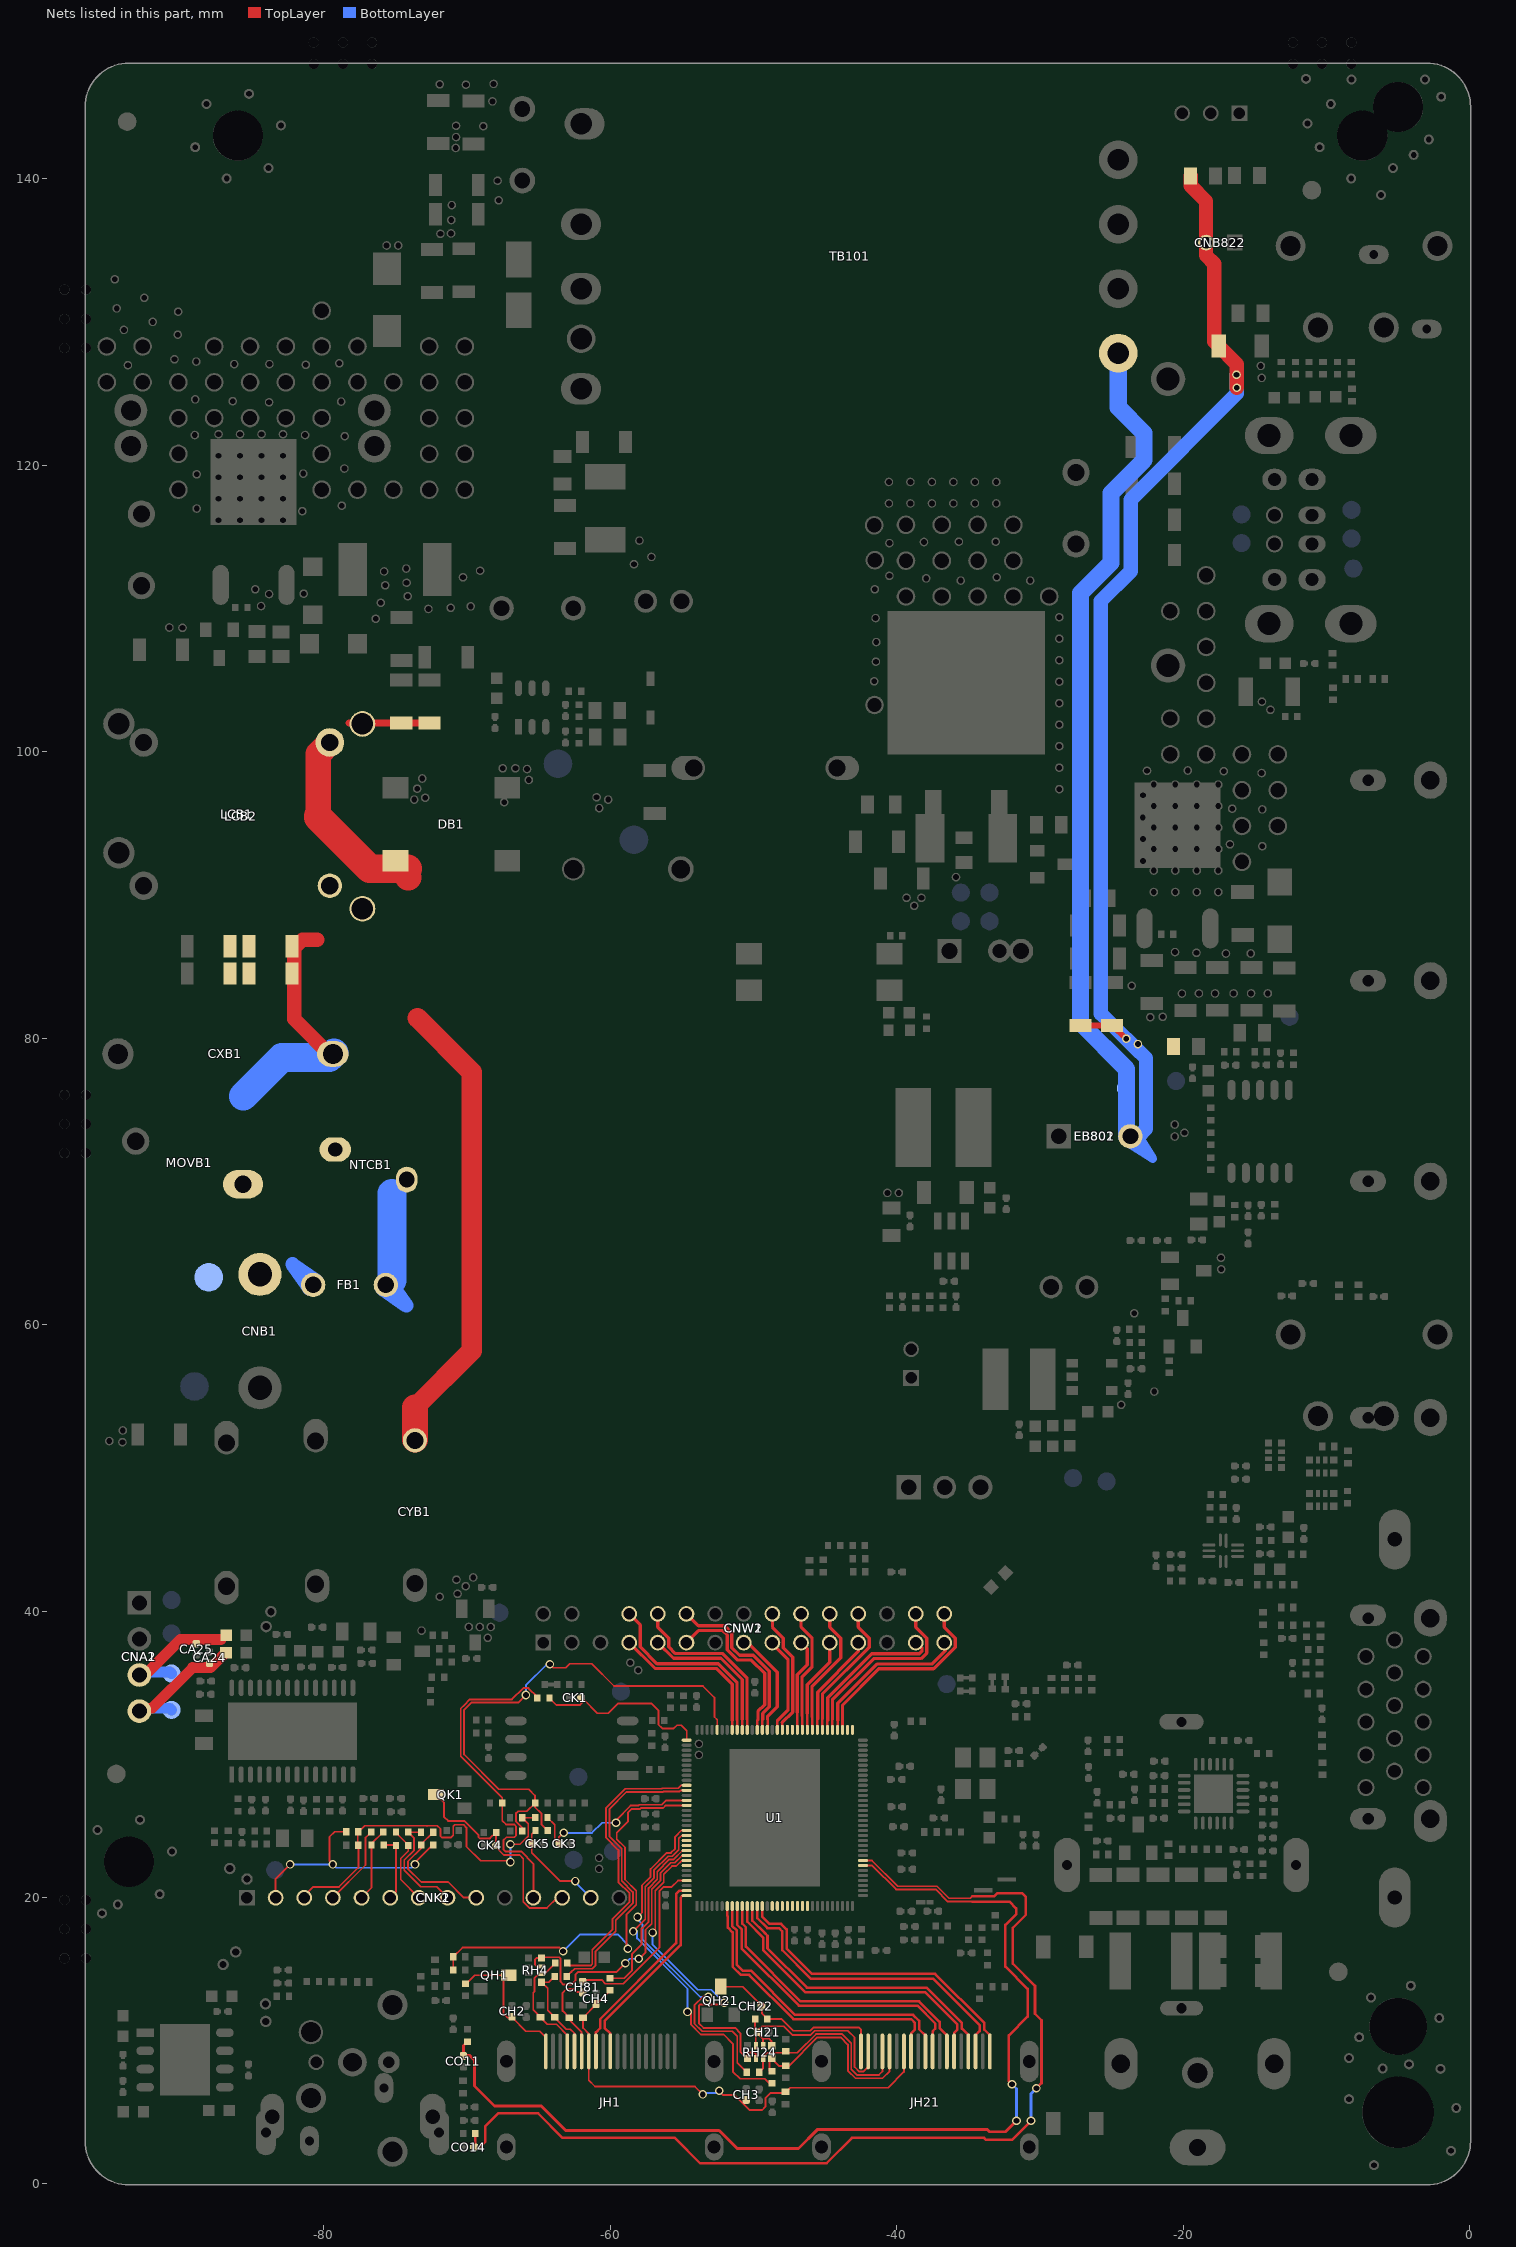
[diagram p0: the nets of this part, all layers, seen from the top]
# Altium PCB MISC86372.PcbDoc (part 11 of 16)
Units mm, origin at the board's own origin, x right, y up, seen from the top; angles counter-clockwise.
Board outline 96.73 x 148.13 mm, 2 copper layers (TopLayer, BottomLayer), stack 1.571 mm thick; 578 components, 318 nets, 2702 pads, 836 vias.

## Via types
v1: diameter 0.6, hole 0.4, TopLayer to BottomLayer, tented both sides, 816 vias
v2: diameter 0.7, hole 0.5, TopLayer to BottomLayer, tented both sides, 15 vias
v3: diameter 0.8, hole 0.5, TopLayer to BottomLayer, tented both sides, 5 vias

## Nets (pads, with @x,y where several pads share a name; then routed paths per layer and width w, separated by ;. In a path a pad name is that pad's centre, name@x,y a point inside that pad or via, vN(x,y) a via of type N, cw(c..) or ccw(c..) an arc to the next point about the centre after c; other vN are vias at no path point) (continued)
HDMI_A_CKN_IN_IC: JH1.12 U1.127 | length 14.1
  TopLayer w0.178: JH1.12@-61,9.258 -61,10.577 -60.706,10.871 -60.706,11.502 -55.397,16.81 -55.397,20.247 -55.188,20.456 -54.687,20.456 U1.127@-54.663,20.481
HDMI_A_CKP_IN_IC: JH1.10 U1.128 | length 13.6
  TopLayer w0.178: JH1.10@-60,9.258 -60,10.495 -60.401,10.897 -60.401,11.375 -55.093,16.684 -55.093,19.981 -54.943,20.131 U1.128@-54.663,20.131
HDMI_A_HPD_OUT: CH2.1 JH1.19 QH1.C RH3.1 | length 10.2
  TopLayer w0.127: RH3.1@-70.098,13.931 -69.463,14.567 QH1.C@-67.081,14.567 ; QH1.C@-67.462,14.185 -67.462,11.911 -67.18,11.628 -66.861,11.628 -65.898,10.665 -64.919,10.665 -64.5,10.247 JH1.19@-64.5,9.258
HDMI_A_HPD_OUT_IC: RH4.2 RH4.4 U1.120 | length 20
  TopLayer w0.127: RH4.4@-64.803,15.185 -65.122,15.185 -65.253,15.316 -65.253,15.676 -65.144,15.785 RH4.2@-64.803,15.785 RH4.2@-64.803,15.909 ; RH4.2@-64.803,15.833 -63.562,15.833 -63.465,15.736 -63.465,14.113 -63.271,13.919 -62.713,13.919 -62.433,14.199 -62.433,14.605 -62.236,14.802 -59.555,14.802 v1(-58.942,15.414) ; v1@-57.991,15.703 -57.551,16.143 -57.551,17.729 -57.099,18.181 -57.099,20.566 -56.497,21.167 -56.497,21.704 -55.775,22.427 -55.488,22.427 -54.984,22.931 U1.120@-54.613,22.931
  BottomLayer w0.127: v1(-58.942,15.414) -58.634,15.723 -58.014,15.723 v1(-58.012,15.724)
HDMI_A_SCL_IN: DH2.K JH1.15 RH4.8 RH6.1 | length 7.1
  TopLayer w0.127: RH6.1@-63.874,14.494 -64.283,14.085 RH4.8@-64.803,14.085 -64.371,13.654 -64.371,12.131 DH2.K@-63.881,11.64 -63.881,11.601 -63.081,10.801 -62.783,10.801 -62.5,10.518 JH1.15@-62.5,9.258
HDMI_A_SCL_IN_IC: RH6.2 U1.107 | length 21.1
  TopLayer w0.127: RH6.2@-63.024,14.494 -62.712,14.807 ; -62.564,14.954 -62.712,14.807 ; U1.107@-54.664,27.481 -55.085,27.481 -55.169,27.397 -56.284,27.397 -56.318,27.364 -58.875,27.364 -60.063,26.175 -60.063,24.265 -59.201,23.403 -59.201,21.161 -58.421,20.381 -58.421,19.599 -59.623,18.397 -59.623,17.655 -61.025,16.252 -61.025,15.261 -61.256,15.03 -62.488,15.03 -62.712,14.807
HDMI_A_SDA_IO: DH3.K JH1.16 RH4.6 RH5.1 | length 8.3
  TopLayer w0.127: RH4.6@-64.99,14.685 -65.287,14.387 -65.287,13.45 -65.38,13.358 -65.38,12.159 DH3.K@-64.861,11.64 ; DH3.K@-64.897,11.645 -64.403,11.151 -63.754,11.151 -63,10.397 JH1.16@-63,9.258 ; RH4.6@-64.803,14.685 -64.587,14.685 RH5.1@-63.855,15.418 RH5.1@-63.932,15.418
HDMI_A_SDA_IO_IC: RH5.2 U1.106 | length 20.8
  TopLayer w0.127: RH5.2@-63.005,15.418 -62.846,15.259 -61.35,15.259 -61.254,15.356 -61.254,16.347 -59.851,17.749 -59.851,18.492 -58.649,19.694 -58.649,20.286 -59.43,21.066 -59.43,23.308 -60.292,24.17 -60.292,26.27 -58.969,27.592 -56.412,27.592 -56.379,27.626 -55.263,27.626 -55.059,27.831 U1.106@-54.664,27.831 ; U1.106@-54.673,27.821 U1.106@-54.663,27.831
HDMI_ARC_OUT: CH81.1 DH81.K JH1.14 | length 6.1
  TopLayer w0.127: DH81.K@-62.865,11.455 -62,10.59 JH1.14@-62,9.258 ; DH81.K@-62.865,11.615 -63.33,12.08 -63.33,13.35 -63.058,13.622 -62.535,13.622 -62.306,13.393 CH81.1@-61.946,13.393
HDMI_ARC_OUT_IC: CH81.2@-61.925,13.995 CH81.2@-61.925,14.17 U1.125 | length 12.7
  TopLayer w0.127: CH81.2@-61.946,14.243 -60.609,14.243 -60.339,13.973 -59.106,13.973 -56.553,16.526 -56.553,20.466 -56.279,20.739 -55.715,20.739 -55.273,21.181 U1.125@-54.663,21.181
HDMI_B_0N_IN_IC: JH21.9 U1.9 | length 20.8
  TopLayer w0.178: U1.9@-51.138,19.406 -51.138,18.099 -50.837,17.797 -50.837,16.451 -46.831,12.446 -38.568,12.446 -37.313,11.191 -37.313,10.846 -37.5,10.658 JH21.9@-37.5,9.258 JH21.9@-37.49,9.267
HDMI_B_0P_IN_IC: JH21.7 U1.10 | length 20.9
  TopLayer w0.178: U1.10@-50.788,19.406 -50.788,18.18 -50.532,17.924 -50.532,16.578 -46.705,12.751 -38.441,12.751 -37.008,11.317 -37.008,10.878 -36.5,10.37 JH21.7@-36.5,9.258 JH21.7@-36.525,9.283
HDMI_B_1N_IN_IC: JH21.6 U1.11 | length 21.2
  TopLayer w0.178: U1.11@-50.438,19.406 -50.438,18.312 -49.33,17.204 -49.33,16.328 -46.401,13.399 -38.036,13.399 -35.763,11.126 -35.763,10.77 -36,10.533 JH21.6@-36,9.258
HDMI_B_1P_IN_IC: JH21.4 U1.12 | length 21.3
  TopLayer w0.178: U1.12@-50.088,19.406 -50.088,18.393 -49.204,17.508 -49.025,17.33 -49.025,16.454 -46.274,13.703 -37.91,13.703 -35.458,11.252 -35.458,10.846 -35,10.387 JH21.4@-35,9.258
HDMI_B_2N_IN_IC: JH21.3 U1.13 | length 22.2
  TopLayer w0.178: U1.13@-49.738,19.406 -49.738,18.569 -49.025,17.856 -48.208,17.856 -47.993,17.641 -47.993,16.32 -46.011,14.338 -37.46,14.338 -34.214,11.092 -34.214,10.671 -34.5,10.385 JH21.3@-34.5,9.258
HDMI_B_2P_IN_IC: JH21.1 U1.14 | length 22.2
  TopLayer w0.178: U1.14@-49.388,19.406 -49.388,18.65 -48.899,18.161 -48.082,18.161 -47.688,17.767 -47.688,16.447 -45.91,14.668 -37.323,14.668 -33.884,11.229 -33.884,10.768 -33.5,10.385 JH21.1@-33.5,9.258
HDMI_B_5V: CH21.1 JH21.18 RH23.2 RH24.4 RH24.6 RH24.8 | length 16.1
  TopLayer w0.127: RH23.2@-49.888,11.527 -49.888,10.74 CH21.1@-49.738,10.59 ; RH24.4@-49.85,9.649 -49.85,10.349 CH21.1@-49.676,10.523 ; CH21.1@-49.809,10.519 CH21.1@-49.738,10.59 ; CH21.1@-49.738,10.394 CH21.1@-49.738,10.59 ; CH21.1@-49.738,10.656 -49.389,11.006 -47.886,11.006 -47.275,10.394 -46.031,10.394 -45.732,10.693 -43.409,10.693 -42.951,10.236 -42.951,8.172 -42.622,7.842 -42.348,7.842 -42,8.19 JH21.18@-42,9.258 ; CH21.1@-49.605,10.398 -49.346,10.138 ; CH21.1@-49.563,10.59 CH21.1@-49.479,10.506 ; RH24.6@-49.35,9.649 -49.346,9.653 -49.346,10.138 ; RH24.8@-48.75,9.649 -48.75,9.974 -48.914,10.138 -49.346,10.138
HDMI_B_CKN_IN_IC: JH21.12 U1.7 | length 20.8
  TopLayer w0.178: U1.7@-51.838,19.406 -51.838,18.734 -51.793,18.689 -51.793,17.892 -51.46,17.559 -51.46,15.164 -50.887,14.591 -50.306,14.591 -47.22,11.506 -38.988,11.506 -38.735,11.253 -38.735,10.77 -39,10.505 JH21.12@-39,9.258
HDMI_B_CKP_IN_IC: JH21.10 U1.8 | length 20.9
  TopLayer w0.178: U1.8@-51.488,19.406 -51.488,18.018 -51.156,17.685 -51.156,15.291 -50.761,14.896 -50.179,14.896 -47.094,11.811 -38.862,11.811 -38.43,11.379 -38.43,10.797 -38,10.367 JH21.10@-38,9.258
HDMI_B_HPD_OUT: CH22.1 JH21.19 QH21.C RH23.1 | length 14.6
  TopLayer w0.127: QH21.C@-52.286,13.768 -50.75,13.768 CH22.1@-49.403,12.421 -49.403,11.892 RH23.1@-49.038,11.527 -48.068,11.527 -47.236,10.696 -46.053,10.696 -45.826,10.922 -45.288,10.922 ; -45.593,10.922 -45.288,10.922 ; JH21.19@-42.5,10.471 JH21.19@-42.5,9.258 -42.5,10.795 -42.627,10.922 -45.288,10.922
HDMI_B_HPD_OUT_IC: RH24.1 RH24.3 U1.121 | length 23.6
  TopLayer w0.127: v1@-56.865,17.551 -56.865,20.477 -56.269,21.073 -56.269,21.61 -55.68,22.198 -55.393,22.198 -55.011,22.581 U1.121@-54.613,22.581 ; v1@-52.007,12.649 v1(-52.045,12.649) -52.045,12.537 -52.056,12.525 -53.75,12.525 -53.816,12.459 -53.816,11.217 -53.491,10.892 -51.278,10.892 -50.913,10.527 -50.913,9.232 RH24.1@-50.43,8.749 -50.43,9.117 -50.374,9.173 -49.905,9.173 -49.83,9.099 RH24.3@-49.83,8.749
  BottomLayer w0.127: v1(-57.048,17.551) -57.048,16.711 -53.901,13.564 -52.959,13.564 v1(-52.045,12.649)
HDMI_B_SCL_IN: DH22.K JH21.15 RH24.7 RH26.1 | length 14.1
  TopLayer w0.127: RH24.7@-48.883,8.745 -48.883,7.87 RH26.1@-48.793,7.78 ; RH24.7@-48.75,8.749 RH24.7@-48.73,8.749 -48.215,8.233 -47.756,8.233 -47.752,8.23 -47.549,8.23 -45.542,10.236 -43.91,10.236 -43.409,9.735 -43.409,7.913 -42.881,7.385 -40.997,7.385 -40.5,7.882 JH21.15@-40.5,9.258
HDMI_B_SCL_IN_IC: RH26.2 U1.116 | length 25.2
  TopLayer w0.127: v1(-58.395,17.63) -57.556,18.468 -57.556,20.755 -56.955,21.357 -56.955,21.894 -55.964,22.884 -55.677,22.884 -55.22,23.341 -55.22,24.127 -55.016,24.331 U1.116@-54.663,24.331 ; v1@-54.356,11.9 -54.356,11.11 -53.68,10.435 -52.076,10.435 -51.435,9.794 -51.435,7.846 -50.929,7.341 -49.204,7.341 RH26.2@-48.793,6.93
  BottomLayer w0.127: v1(-58.395,17.63) -58.129,17.63 -58.129,17.145 -54.61,13.626 v1(-54.61,12.014)
HDMI_B_SDA_IO: DH23.K JH21.16 RH24.5 RH25.1 | length 13.9
  TopLayer w0.127: RH25.1@-49.613,7.798 -49.33,8.081 RH24.5@-49.33,8.749 -49.33,8.882 -49.049,9.164 -46.946,9.164 -46.942,9.16 -45.637,10.465 -43.815,10.465 -43.18,9.83 -43.18,8.008 -42.786,7.614 -41.241,7.614 -41,7.855 JH21.16@-41,9.258
HDMI_B_SDA_IO_IC: RH25.2 U1.115 | length 24.2
  TopLayer w0.127: v1(-58.092,18.642) -57.785,18.948 -57.785,20.85 -57.183,21.452 -57.183,21.989 -56.059,23.113 -55.772,23.113 -55.474,23.411 -55.474,24.232 -55.026,24.681 U1.115@-54.663,24.681 ; v1@-53.365,13.106 -53.492,13.106 -54.127,12.471 -54.127,11.205 -53.586,10.663 -51.481,10.663 -51.142,10.324 -51.142,8.477 RH25.2@-50.463,7.798
  BottomLayer w0.127: v1(-58.092,18.642) -58.092,18.468 -57.76,18.136 -57.76,17.099 -53.716,13.056 v1(-53.162,13.056)
HDMI_C_0N_IN_IC: U1.18
HDMI_C_0P_IN_IC: U1.19
HDMI_C_1N_IN_IC: U1.20
HDMI_C_1P_IN_IC: U1.21
HDMI_C_2N_IN_IC: U1.22
HDMI_C_2P_IN_IC: U1.23
HDMI_C_CKN_IN_IC: U1.16
HDMI_C_CKP_IN_IC: U1.17
HDMI_C_HPD_OUT_IC: U1.122
HDMI_C_SCL_IN_IC: U1.118
HDMI_C_SDA_IO_IC: U1.117
HDMI_CEC_IO: CH3.2@-50.506,5.819 CH3.2@-50.506,5.994 CH4.2@-61.006,12.503 CH4.2@-61.006,12.678 DH1.K DH21.K JH1.13 JH21.13 RH83.2 | length 34.3
  TopLayer w0.127: CH4.2@-61.006,12.503 -60.02,13.489 RH83.2@-60.02,13.513 ; CH4.2@-61.006,12.515 DH1.K@-61.906,11.615 -61.906,10.895 -61.5,10.489 JH1.13@-61.5,9.258 -61.5,7.239 -61.068,6.807 -54.092,6.807 v1(-53.538,6.253) ; v1@-52.4,6.477 -52.146,6.223 -51.353,6.223 -50.301,5.171 -49.397,5.171 -49.393,5.167 -49.174,5.386 -49.174,5.989 -48.822,6.342 -47.802,6.342 -47.422,6.722 -40.598,6.722 -39.5,7.82 JH21.13@-39.5,9.258 JH21.13@-39.5,10.392
  BottomLayer w0.127: v1(-53.538,6.253) -53.441,6.35 -52.553,6.35 v1(-52.4,6.502)
HDMI_CEC_IO_IC: RH83.1 U1.119 | length 12.1
  TopLayer w0.127: RH83.1@-60.02,14.363 -59.039,14.363 -58.477,14.924 -58.477,16.06 -57.81,16.727 -57.81,17.831 -57.328,18.313 -57.328,20.66 -56.726,21.262 -56.726,21.799 -55.87,22.656 -55.583,22.656 -54.958,23.281 U1.119@-54.613,23.281
HDMI_DET: RH81.1 RH82.1 U1.110 | length 29.5
  TopLayer w0.127: RH82.1@-70.961,15.861 -70.312,16.51 -63.551,16.51 ; RH82.1@-70.923,15.823 -70.961,15.785 RH81.1@-70.961,14.935 ; -63.525,16.51 -63.551,16.51 ; v1(-63.297,16.256) -63.551,16.51 ; v1@-58.86,16.516 -58.86,18.837 -58.192,19.504 -58.192,20.475 -58.972,21.256 -58.972,23.497 -59.55,24.075 -59.55,24.519 -58.768,25.3 -58.768,25.914 -58.496,26.187 -57.914,26.187 -57.853,26.247 -56.298,26.247 -56.114,26.431 U1.110@-54.664,26.431 ; RH81.1@-70.961,14.935 -70.961,14.884 RH81.1@-70.961,14.935
  BottomLayer w0.127: v1@-63.246,16.29 -62.111,17.424 -59.493,17.424 -58.769,16.701 v1(-58.769,16.426)
IR_IN: CNK1.11 CNK2.11 RK1.1 RK2.1 | length 24.2
  TopLayer w0.127: -67.749,27.17 -68.162,27.584 ; CNK2.11@-65.365,19.99 -65.365,22.362 -66.222,23.22 -67.322,23.22 -67.462,23.36 -67.462,23.991 -67.246,24.207 -66.694,24.207 -66.583,24.319 -66.583,24.971 -66.717,25.104 -67.279,25.104 -67.545,25.371 RK1.1@-67.545,26.594 -67.545,26.967 -68.162,27.584 ; RK2.1@-65.093,33.925 -65.093,34.001 -65.712,34.62 -66.077,34.62 -66.865,33.833 -68.274,33.833 -68.275,33.831 -69.801,33.831 -70.21,33.422 -70.437,33.195 -70.437,29.858 -68.162,27.584
IR_IN_IC: CK1.2@-62.014,33.941 CK1.2@-62.189,33.941 RK2.2 U1.97 | length 12.9
  TopLayer w0.127: RK2.2@-64.243,33.925 -63.753,33.435 -62.122,33.435 -62.014,33.543 -62.014,33.905 CK1.2@-62.014,33.941 ; CK1.2@-61.836,33.801 -60.902,32.868 -60.138,32.868 -59.452,33.553 -57.134,33.553 -56.642,33.062 -56.642,32.076 -56.367,31.801 -55.573,31.801 -55.344,32.029 -55.044,32.029 -54.664,31.649 U1.97@-54.664,30.981
K0: CNK1.9 CNK2.9 RK7.1 RK8.2 | length 8.8
  TopLayer w0.127: RK7.1@-73.225,23.7 RK8.2@-72.366,24.559 ; RK7.1@-73.207,23.663 -73.207,23.431 -74.126,22.512 -74.126,22.012 -73.196,21.082 -71.323,21.082 -70.231,19.99 CNK2.9@-69.365,19.99
K1: CNK1.8 CNK2.8 RK8.1 RK9.2 | length 7.8
  TopLayer w0.127: RK9.2@-74.11,24.567 RK9.2@-74.102,24.559 ; RK8.1@-73.216,24.559 RK9.2@-74.102,24.559 ; CNK2.8@-71.365,19.99 -72.127,20.752 -73.225,20.752 -74.38,21.906 -74.38,22.617 -73.694,23.303 -73.694,24.151 RK9.2@-74.102,24.559
K2: CNK1.7 CNK2.7 RK9.1 RK11.2 | length 5.7
  TopLayer w0.127: RK9.1@-74.96,24.567 -74.96,24.508 RK11.2@-74.085,23.633 ; RK11.2@-74.109,23.641 -74.109,23.247 -74.634,22.723 -74.634,21.259 CNK2.7@-73.365,19.99
K3: CNK1.6 CNK2.6 RK11.1 RK12.2 | length 4.8
  TopLayer w0.127: RK12.2@-75.821,23.658 RK11.1@-74.997,23.658 ; CNK2.6@-75.365,19.99 -74.959,20.395 RK11.1@-74.959,23.743 ; RK11.1@-74.97,23.631 RK11.1@-74.959,23.62
K4: CNK1.5 CNK2.5 RK12.1 RK16.2 | length 5.3
  TopLayer w0.127: CNK2.5@-77.365,19.99 -76.671,20.683 RK12.1@-76.671,23.76 ; RK12.1@-76.675,23.658 -76.675,23.748 RK16.2@-75.85,24.573
K5: CNK1.4 CNK2.4 RK16.1 | length 5.7
  TopLayer w0.127: CNK2.4@-79.365,19.99 -77.087,22.268 -77.087,24.186 RK16.1@-76.7,24.573
K6: CNK1.3 CNK2.3 DK1.K RK3.1 RK4.2 RK6.2 | length 26.4
  TopLayer w0.127: CNK2.3@-81.365,19.99 -81.365,20.108 -80.734,20.739 -78.939,20.739 -77.585,22.093 DK1.K@-77.585,23.648 ; DK1.K@-77.627,23.582 -77.627,24.539 -77.152,25.013 -72.806,25.013 ; -72.773,24.999 -72.792,24.999 -72.806,25.013 ; v1@-66.972,22.563 -69.053,22.563 -70.036,23.546 -70.04,23.546 -70.04,24.881 -70.243,25.084 -70.861,25.084 -70.958,24.987 -70.958,24.343 -71.107,24.194 -71.753,24.194 -71.851,24.292 -71.851,24.789 -72.076,25.013 -72.806,25.013 ; v1(-66.972,23.717) -66.301,23.717 -65.733,24.285 -65.733,25.152 RK3.1@-66.15,25.569 -65.249,25.569 RK4.2@-65.233,25.585
  BottomLayer w0.127: v1(-66.972,22.475) v1(-66.972,23.717)
K7: CNK1.2 CNK2.2 RK6.1 RK7.2 | length 17.2
  TopLayer w0.127: CNK2.2@-83.138,19.99 CNK2.2@-83.365,19.99 -83.365,21.296 v1(-82.352,22.309) ; v1(-79.367,22.309) -79.604,22.546 -79.604,24.232 -79.24,24.595 RK6.1@-78.433,24.595 ; v1@-73.661,22.322 -73.661,22.42 RK7.2@-72.327,23.754
  BottomLayer w0.127: v1(-82.352,22.309) v1(-79.367,22.309) -79.131,22.073 -73.872,22.073 v1(-73.635,22.309)
KEY_IN_IC: CK3.2@-63.42,23.749 CK3.2@-63.595,23.749 RK4.1 U1.109 | length 12.5
  TopLayer w0.127: RK4.1@-64.383,25.585 -63.881,25.082 -63.881,24.035 CK3.2@-63.595,23.749 -63.595,24.218 v1@-63.274,24.539 ; v1@-59.598,25.408 -58.591,26.415 -58.034,26.415 -57.973,26.475 -56.392,26.475 -56.087,26.781 U1.109@-54.664,26.781
  BottomLayer w0.127: v1(-63.246,24.511) -61.28,24.511 -60.57,25.221 v1(-59.598,25.221)
L: CYB1.1 DB1.2 LCB1.3 LCB2.3 RB101.1 RB141.2 | length 51.6
  TopLayer w0.5: -78.224,101.989 -78.208,102.005 RB141.2@-72.619,102.005
  TopLayer w1.4: -73.635,54.204 -69.672,58.166 -69.672,77.622 -73.457,81.407
  TopLayer w1.8: -80.391,95.504 -80.391,99.822 LCB1.3@-79.578,100.635 ; -74.131,91.201 -74.08,91.201 ; CYB1.1@-73.635,51.968 -73.635,54.204
  TopLayer w2: -80.391,95.504 -80.391,95.409 -76.793,91.811 DB1.2@-74.131,91.811
L-1: CNB1.1 FB1.1 TP_L.1
L-2: FB1.2 NTCB1.1 | length 6.1
  BottomLayer w2: FB1.2@-75.235,63.094 -75.235,69.164
L-3: CXB1.1 LCB1.2 LCB2.2 MOVB1.1 NTCB1.2@-79.208,72.221 RB1.1 RB2.1 | length 18.3
  TopLayer w1: -80.467,86.868 -81.483,86.868 -82.067,86.284 -82.067,81.331 CXB1.1@-79.299,78.562
  BottomLayer w2: -85.633,75.937 -82.931,78.638 -79.622,78.638 CXB1.1@-79.292,78.969
L-N: RB1.2 RB2.2 RB3.1 RB4.1
LED_FB: CB808.2 CNB822.2 EB801.2 EB802.2@-23.687,73.139 pad.VIA5@-16.256,125.4 pad.VIA5@-16.281,126.314 pad.VIA5@-23.165,79.578 pad.VIA5@-23.978,79.959 RB814.1 RB825.2 RB826.2 RB845.1 TB101.7 TP_LED-.1 | length 138.8
  TopLayer w0.4: RB826.2@-27.178,80.796 -27.102,80.872 RB825.2@-24.968,80.872 pad.VIA5@-23.978,79.959
  TopLayer w1: RB845.1@-19.484,140.183 -19.484,139.499 -18.408,138.423 CNB822.2@-18.408,135.534 -18.408,135.299 -18.408,134.639 -17.831,134.061 -17.831,128.623 CB808.2@-17.527,128.32 -16.256,127.048 pad.VIA5@-16.256,125.4
  BottomLayer w1: pad.VIA5@-23.978,79.959 -22.606,78.588 -22.606,73.66 -23.113,73.153 -23.127,73.139 EB801.2@-23.687,73.139 ; -23.087,79.039 -25.756,81.708 -25.756,110.515 -23.673,112.598 -23.673,117.577 -16.256,124.993 pad.VIA5@-16.256,125.4 pad.VIA5@-16.256,126.314
  BottomLayer w1.2: TB101.7@-24.538,127.819 -24.538,124.03 -22.733,122.225 -22.733,120.345 -25.044,118.034 -25.044,113.182 -27.178,111.049 -27.178,81.051 -23.952,77.826 EB801.2@-23.952,73.139
LED_G: CK4.1 CNK1.12 CNK2.12 QK1.C RK10.1 | length 16.4
  TopLayer w0.127: QK1.C@-72.162,27.191 -71.598,26.626 -71.598,25.617 -71.325,25.345 -70.688,25.345 ; -71.209,25.345 -70.688,25.345 ; CK4.1@-68.054,23.601 CK4.1@-67.97,23.518 ; RK10.1@-67.97,24.544 CK4.1@-67.97,23.518 ; RK10.1@-67.962,24.575 -68.407,24.129 -69.114,24.129 -69.211,24.226 -69.211,24.374 -70.181,25.345 -70.688,25.345 ; CNK2.12@-63.365,19.99 -63.703,19.99 -64.418,19.275 -65.661,19.275 -66.08,19.694 -66.08,22.718 -66.327,22.966 -67.427,22.966 -67.97,23.509 CK4.1@-67.97,23.518
LED_OUT_IC: RK13.1 RK14.2 RK15.2 U1.92 | length 38.1
  TopLayer w0.127: -68.084,33.604 -68.021,33.604 ; RK15.2@-66.148,24.648 -66.148,24.859 -66.575,25.286 -66.575,25.889 -66.438,26.025 -65.822,26.025 RK13.1@-65.254,26.594 ; v1(-65.888,34.138) -66.421,33.604 -68.021,33.604 ; -65.783,27.559 -65.989,27.559 ; RK14.2@-64.37,24.666 -64.808,25.104 -64.808,25.868 -65.254,26.313 RK13.1@-65.254,26.594 ; v1(-64.216,36.279) -63.979,36.043 -63.119,36.043 -62.84,36.322 -61.297,36.322 -59.738,34.763 -53.532,34.763 -52.723,33.954 -52.723,32.599 -52.538,32.414 U1.92@-52.538,31.707 ; U1.92@-52.538,31.656 U1.92@-52.538,31.707 ; -68.021,33.604 -68.023,33.603 -69.706,33.603 -70.208,33.101 -70.208,29.985 -67.782,27.559 -65.989,27.559 ; -65.989,27.559 -65.694,27.559 -65.254,27.118 RK13.1@-65.254,26.594
  BottomLayer w0.127: v1(-65.888,34.138) -65.888,34.81 -64.418,36.279 v1(-64.216,36.279)
LED_R: CK5.1 CNK1.13 CNK2.13 RK14.1 | length 7.1
  TopLayer w0.127: CK5.1@-65.227,23.752 CK5.1@-65.22,23.759 ; RK14.1@-65.22,24.666 -65.479,24.408 -65.479,23.754 CK5.1@-65.481,23.752 -65.481,23.132 -63.495,21.145 v1(-62.453,21.145)
  BottomLayer w0.127: v1(-62.453,21.145) -62.453,21.079 CNK2.13@-61.365,19.99
LINE_L_OUT_IC: CO11.2@-70.256,8.81 CO11.2@-70.256,8.985 RO12.2 U1.39 | length 72.8
  TopLayer w0.127: U1.39@-42.362,22.231 -41.712,22.231 -40.043,20.561 -37.286,20.561 -36.439,19.715 -34.744,19.715
  TopLayer w0.178: -34.744,19.715 -32.143,19.715 -31.666,19.237 ; v1(-31.953,6.96) -32.177,7.184 -32.177,10.368 -30.858,11.688 -30.858,13.619 -32.41,15.172 -32.41,18.082 -31.666,18.827 -31.666,19.237 ; -31.674,19.245 -31.666,19.237
  TopLayer w0.203: RO12.2@-69.977,9.938 -70.256,9.659 CO11.2@-70.256,8.985 -69.818,8.985 -69.475,8.642 -69.475,6.844 -68.079,5.448 -64.814,5.448 -63.109,3.743 -52.397,3.743 -51.897,3.243 ; -51.897,3.239 -51.134,2.476 -46.87,2.476 -45.557,3.789 -33.667,3.789 -33.526,3.648 -32.401,3.648 -31.641,4.408 v1(-31.641,4.414)
  BottomLayer w0.178: v1(-31.953,6.96) -31.641,6.647 v1(-31.641,4.414)
LINE_R_OUT_IC: CO14.2@-69.462,2.577 CO14.2@-69.637,2.577 RO15.2 U1.40 | length 73.9
  TopLayer w0.127: U1.40@-42.362,22.581 -41.729,22.581 -39.938,20.79 -37.191,20.79 -36.353,19.952 -34.866,19.952 -34.727,20.091
  TopLayer w0.178: CO14.2@-69.637,2.577 -69.085,2.577 -68.713,2.948 -68.713,4.045 -67.831,4.928 -65.03,4.928 -63.325,3.222 -55.496,3.222 -53.721,1.448 -52.743,1.448 -44.903,1.448 -43.134,3.218 -33.904,3.218 -33.763,3.077 -31.943,3.077 v1@-30.629,4.39 ; -34.727,20.091 -33.191,20.091 -32.97,20.312 -31.255,20.312 -30.98,20.038 -30.98,18.794 -31.902,17.872 -31.902,15.382 -30.35,13.83 -30.35,11.883 -29.896,11.429 -29.896,7.036 v1(-30.251,6.68)
  TopLayer w0.203: CO14.2@-69.425,2.577 RO15.2@-69.425,3.516 ; v1@-30.629,4.39 v1(-30.629,4.414)
  BottomLayer w0.203: -30.629,4.739 -30.629,6.302 v1(-30.251,6.68)
LOUT+: BA1.2 CA24.2@-87.979,36.326 CA24.2@-87.979,36.501 CNA1.4 CNA2.4 LOUT+.1 | length 10
  TopLayer w0.762: CNA1.4@-92.877,33.213 -91.983,33.213 -89.153,36.044 -87.905,36.044 BA1.2@-86.827,37.122
  BottomLayer w0.762: CNA1.4@-92.877,33.213 -90.744,33.213 LOUT+.1@-90.627,33.096
LOUT-: BA2.2 CA25.1 CNA1.3 CNA2.3 LOUT-.1 | length 9
  TopLayer w0.762: CNA1.3@-92.877,35.533 -92.483,35.533 -90.003,38.013 BA2.2@-87.175,38.013
  BottomLayer w0.762: CNA1.3@-92.877,35.733 -90.724,35.733 LOUT-.1@-90.627,35.636
LVDS_E0N_IC: CNW1.19 CNW2.19 U1.76 | length 7.2
  TopLayer w0.178: U1.76@-46.938,31.707 -46.938,33.243
  TopLayer w0.229: -46.939,32.918 -46.939,35.542 -46.246,36.235 -46.246,37.361 CNW2.19@-46.682,37.796 CNW2.19@-46.374,37.796
LVDS_E0P_IC: CNW1.20 CNW2.20 U1.75 | length 8.7
  TopLayer w0.178: -46.609,32.69 -46.588,32.669 U1.75@-46.588,31.707
  TopLayer w0.229: CNW2.20@-46.682,39.796 -46.682,38.879 -45.916,38.114 -45.916,36.098 -46.609,35.405 -46.609,32.69
LVDS_E1N_IC: CNW1.21 CNW2.21 U1.74 | length 7.8
  TopLayer w0.178: U1.74@-46.238,31.707 -46.238,32.832
  TopLayer w0.229: -46.253,32.842 -46.253,34.856 -44.681,36.428 ; CNW2.21@-44.681,37.428 -44.681,36.428 ; CNW2.21@-44.591,37.796 CNW2.21@-44.681,37.796 -44.681,36.428
LVDS_E1P_IC: CNW1.22 CNW2.22 U1.73 | length 9.4
  TopLayer w0.178: U1.73@-45.888,31.707 -45.888,32.751
  TopLayer w0.229: -45.923,32.614 -45.923,34.719 -43.916,36.727 -43.916,37.479 -43.916,38.114 -44.681,38.879 CNW2.22@-44.681,39.796
LVDS_E2N_IC: CNW1.23 CNW2.23 U1.72 | length 7.5
  TopLayer w0.178: U1.72@-45.538,31.707 -45.538,32.67
  TopLayer w0.229: -45.517,32.461 -45.517,34.345 -42.681,37.18 CNW2.23@-42.681,37.796
LVDS_E2P_IC: CNW1.24 CNW2.24 U1.71 | length 9.9
  TopLayer w0.178: U1.71@-45.188,31.707 -45.188,32.589
  TopLayer w0.229: -45.187,32.461 -45.187,34.208 -41.916,37.479 -41.916,38.114 -42.681,38.879 CNW2.24@-42.681,39.796
LVDS_E3N_IC: CNW1.29 CNW2.29 U1.68 | length 10.9
  TopLayer w0.178: U1.68@-44.138,31.707 U1.68@-44.124,31.72 ; -44.124,32.302 U1.68@-44.124,31.72 ; U1.68@-44.114,31.706 -44.124,31.715 U1.68@-44.124,31.72
  TopLayer w0.229: -44.118,32.36 -44.118,33.564 -41.386,36.297 -37.565,36.297 CNW2.29@-36.594,37.268
LVDS_E3P_IC: CNW1.30 CNW2.30 U1.67 | length 13.9
  TopLayer w0.178: U1.67@-43.788,31.707 -43.788,32.614
  TopLayer w0.229: -43.788,32.614 -43.788,33.428 -41.25,35.966 -37.428,35.966 -35.916,37.479 -35.916,38.114 -36.681,38.879 CNW2.30@-36.681,39.796
LVDS_E4N_IC: U1.66
LVDS_E4P_IC: U1.65
LVDS_ECKN_IC: CNW1.27 CNW2.27 U1.70 | length 10.9
  TopLayer w0.178: U1.70@-44.838,31.707 -44.838,32.314
  TopLayer w0.229: -44.818,32.36 -44.818,33.947 -41.758,37.008 -39.437,37.008 -38.437,37.008 -38.246,37.199 -38.246,37.45 -38.592,37.796 CNW2.27@-38.681,37.796
LVDS_ECKP_IC: CNW1.28 CNW2.28 U1.69 | length 13.1
  TopLayer w0.178: U1.69@-44.488,31.707 -44.488,32.427
  TopLayer w0.229: -44.488,32.427 -44.488,33.81 -41.621,36.678 -38.301,36.678 -37.916,37.063 -37.916,38.114 -38.681,38.879 CNW2.28@-38.681,39.796
LVDS_O0N_IC: CNW1.7 CNW2.7 U1.89 | length 11.6
  TopLayer w0.178: U1.89@-51.488,31.707 -51.488,32.383
  TopLayer w0.229: CNW2.7@-58.682,37.796 -56.877,35.992 -52.587,35.992 -51.488,34.893 -51.488,32.383
LVDS_O0P_IC: CNW1.8 CNW2.8 U1.88 | length 14.9
  TopLayer w0.178: U1.88@-51.138,31.707 -51.138,32.418
  TopLayer w0.229: CNW2.8@-58.682,39.796 -57.916,39.03 ; -57.916,37.866 -57.916,39.03 ; -51.158,32.418 -51.158,35.03 -52.45,36.322 -56.74,36.322 -57.916,37.497 -57.916,39.03
LVDS_O1N_IC: CNW1.9 CNW2.9 U1.87 | length 10.5
  TopLayer w0.178: U1.87@-50.788,31.707 -50.788,32.445
  TopLayer w0.229: CNW2.9@-56.681,37.796 -55.585,36.7 -52.27,36.7 -50.788,35.218 -50.788,32.445
LVDS_O1P_IC: CNW1.10 CNW2.10 U1.86 | length 12.6
  TopLayer w0.178: U1.86@-50.438,31.707 -50.438,32.445
  TopLayer w0.229: CNW2.10@-56.681,39.796 -56.681,38.879 -55.916,38.114 -55.916,37.497 -55.449,37.03 -52.134,37.03 -50.458,35.355 -50.458,32.445
LVDS_O2N_IC: CNW1.11 CNW2.11 U1.84 | length 11.8
  TopLayer w0.178: U1.84@-49.738,31.707 -49.738,32.365 -49.693,32.41
  TopLayer w0.229: CNW2.11@-54.681,37.796 -53.844,38.633 -52.146,38.633 -51.841,38.329 -51.841,37.303 -51.115,36.576 -50.149,36.576 -49.225,35.652 -49.225,35.331 -49.225,33.457 -49.693,32.989 -49.693,32.41
LVDS_O2P_IC: CNW1.12 CNW2.12 U1.83 | length 12.3
  TopLayer w0.178: U1.83@-49.388,31.707 -49.388,32.445
  TopLayer w0.229: CNW2.12@-54.681,39.796 -53.849,38.964 -52.009,38.964 -51.511,38.465 -51.511,37.44 -50.978,36.906 -50.013,36.906 -48.895,35.789 -48.895,33.32 -49.363,32.852 -49.363,32.445
LVDS_O3N_IC: CNW1.17 CNW2.17 U1.80 | length 6.8
  TopLayer w0.178: U1.80@-48.338,31.707 -48.338,32.377
  TopLayer w0.229: CNW2.17@-48.682,37.796 -48.682,37.722 -47.6,36.64 -47.6,33.081 -48.303,32.377
LVDS_O3P_IC: CNW1.18 CNW2.18 U1.79 | length 9
  TopLayer w0.178: U1.79@-47.988,31.707 -47.988,32.225
  TopLayer w0.229: CNW2.18@-48.682,39.796 -48.682,38.879 -47.916,38.114 -47.916,37.423 -47.269,36.777 -47.269,32.944 -47.988,32.225
LVDS_O4N_IC: U1.78
LVDS_O4P_IC: U1.77
LVDS_OCKN_IC: CNW1.15 CNW2.15 U1.82 | length 7.5
  TopLayer w0.178: U1.82@-49.038,31.707 -49.014,31.73 -49.014,32.231 -49.004,32.24 -49.004,32.436
  TopLayer w0.229: CNW2.15@-50.65,37.828 -50.445,37.828 -50.058,37.441 -48.336,35.719 -48.336,33.304 -49.03,32.611 -49.03,32.436